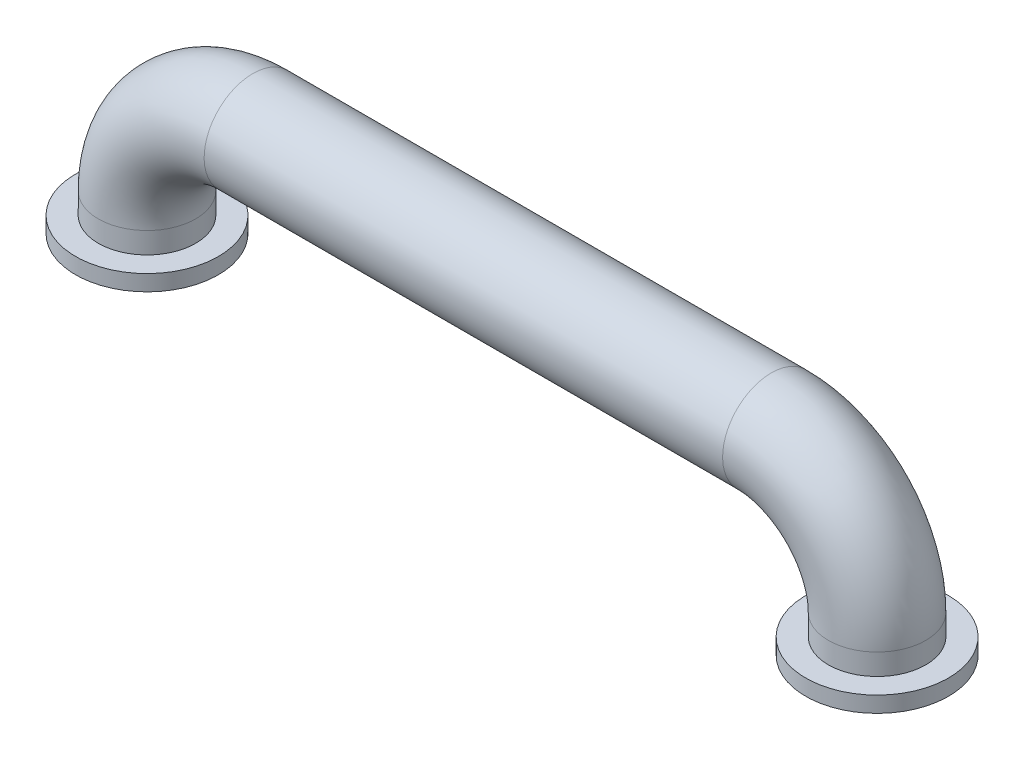
from build123d import *
from build123d.topology import SkipClean

# Parameters (mm, degrees)
SKETCH2_R           = 46
SKETCH2_R_2         = 40
SKETCH4_R           = 67.5
SKETCH4_R_2         = 40
BOSS_EXTRUDE1_DEPTH = 15


with BuildPart() as part:
    # Sweep1: sweep along a path in Sketch3
    with BuildLine(Plane.XY) as sweep1_path:
        Line((0, 0), (0, 20))
        ThreePointArc((0, 20), (29.289321881, 90.710678119), (100, 120))
        Line((100, 120), (590, 120))
        ThreePointArc((590, 120), (660.710678119, 90.710678119), (690, 20))
        Line((690, 20), (690, 0))
    # Sketch2 → Sweep1 (sweep)
    with BuildSketch(Plane(origin=(0, 0, 0), x_dir=(1, 0, 0), z_dir=(0, 1, 0))):
        Circle(SKETCH2_R)
        Circle(SKETCH2_R_2, mode=Mode.SUBTRACT)
    sweep(path=sweep1_path.line)

    # Sketch4 → Boss-Extrude1 (add)
    # profile 1 of 2: a face of its own
    with SkipClean():  # the faces are left unmerged after this step: merging them gives an invalid solid
        with BuildSketch(Plane(origin=(0, 0, 0), x_dir=(-1, 0, 0), z_dir=(0, -1, 0))):
            with Locations(Location((0, 0, 0), (0, 0, 90))):
                Circle(SKETCH4_R)
            Circle(SKETCH4_R_2, mode=Mode.SUBTRACT)
        # profile 2 of 2: a face of its own
        with BuildSketch(Plane(origin=(0, 0, 0), x_dir=(-1, 0, 0), z_dir=(0, -1, 0))):
            with Locations(Location((-690, 0, 0), (0, 0, 90))):
                Circle(SKETCH4_R)
            with Locations(Location((-690, 0, 0), (0, 0, 90))):
                Circle(SKETCH4_R_2, mode=Mode.SUBTRACT)
        extrude(amount=BOSS_EXTRUDE1_DEPTH)


solid = part.part
